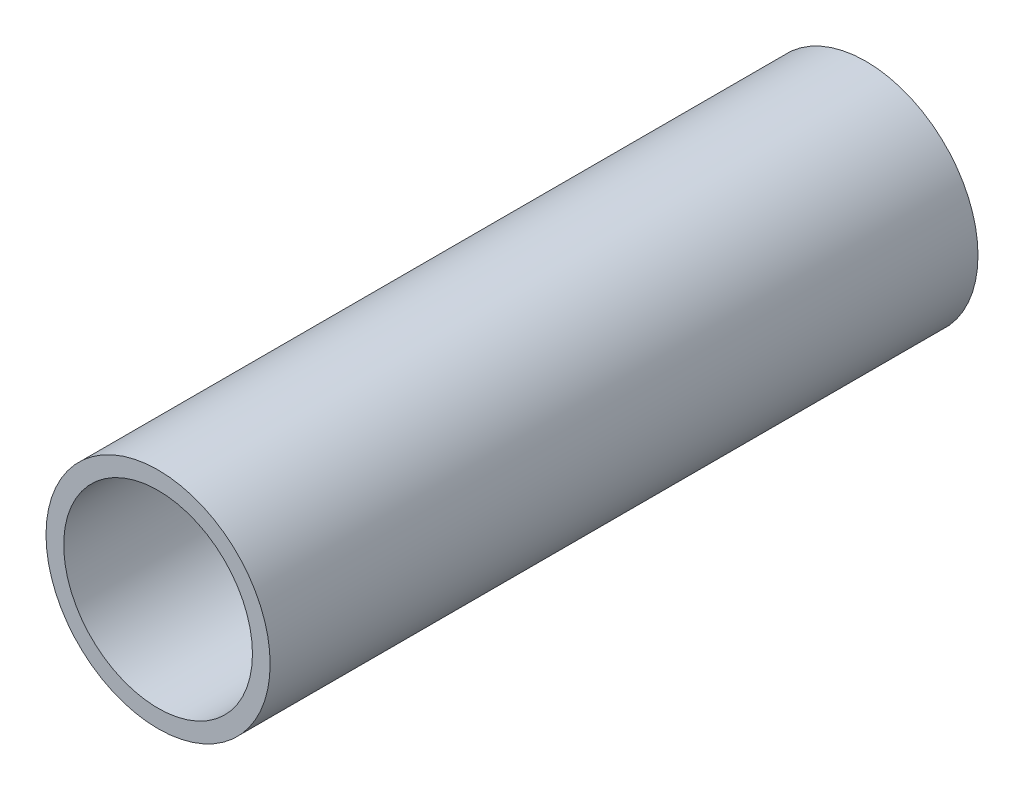
SolidWorks part; units mm, degrees
ref_plane "Front Plane" through (0, 0, 0) normal (0, 0, 1) x (1, 0, 0)
ref_plane "Top Plane" through (0, 0, 0) normal (0, 1, 0) x (1, 0, 0)
ref_plane "Right Plane" through (0, 0, 0) normal (1, 0, 0) x (0, 0, -1)
sketch "Sketch1" plane through (0, 0, 0) normal (0, 0, 1) x (1, 0, 0)
  circle A0 centre (0, 0) radius 2.413
  circle A1 centre (0, 0) radius 2.032
  dimension "D1" = 4.826
  dimension "D2" = 4.064
extrude "Boss-Extrude1" add sketch "Sketch1" against normal blind 15.24
scale "Scale1" bodies to scale 101 scale about origin uniform scaling yes scale factor 2
